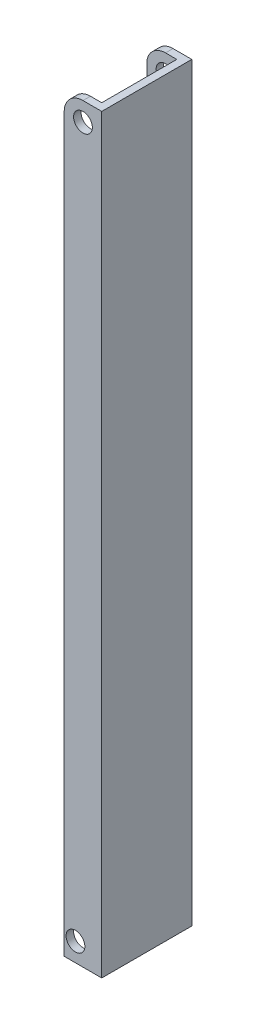
SolidWorks part; units mm, degrees
ref_plane "Front Plane" through (0, 0, 0) normal (0, 0, 1) x (1, 0, 0)
ref_plane "Top Plane" through (0, 0, 0) normal (0, 1, 0) x (1, 0, 0)
ref_plane "Right Plane" through (0, 0, 0) normal (1, 0, 0) x (0, 0, -1)
other "Configuration Table"
ref_plane "Plane1" through (0, 50, 0) normal (0, 1, 0) x (1, 0, 0)
sketch "Sketch2" plane through (0, 50, 0) normal (0, 1, 0) x (1, 0, 0)
  line L0 (35, 10) -> (35, 20)
  line L1 (35, 20) -> (35, 0) construction
  line L2 (35, 20) -> (27, 20)
  line L3 (35, 20) -> (22.9129, 20) construction
  line L4 (27, 20) -> (27, 22)
  line L5 (27, 22) -> (37, 22)
  line L6 (37, 22) -> (37, -2)
  line L7 (37, -2) -> (27, -2)
  line L8 (27, -2) -> (27, 0)
  line L9 (27, 0) -> (35, 0)
  line L10 (35, 0) -> (35, 10)
  dimension "D1" = 2
  dimension "D2" = 2
  dimension "D3" = 2
  dimension "D4" = 10
extrude "Boss-Extrude1" add sketch "Sketch2" along normal blind 200
sketch "Sketch3" plane through (0, 0, 2) normal (0, 0, 1) x (1, 0, 0)
  line L0 (27, 250) -> (27, 50) construction
  line L2 (27, 50) -> (37, 50) construction
  circle A0 centre (30, 55) radius 2.5
  dimension "D1" = 5
  dimension "D2" = 3
  dimension "D3" = 5
extrude "Cut-Extrude1" cut sketch "Sketch3" against normal through all both and the other way through all
fillet "Fillet1" radius 5 2 edges at (27, 250, -21) (27, 250, 1)
sketch "Sketch5" plane through (0, 0, 2) normal (0, 0, 1) x (1, 0, 0)
  circle A0 centre (32, 245) radius 2.5
  dimension "D1" = 5
extrude "Cut-Extrude2" cut sketch "Sketch5" against normal through all both
